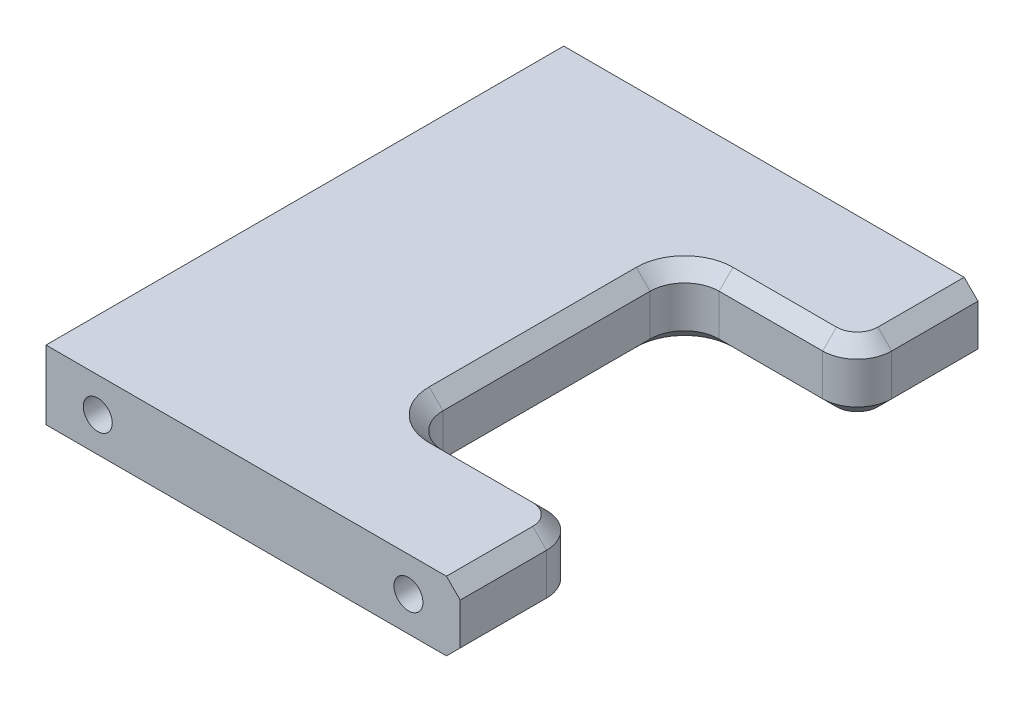
SolidWorks part; units mm, degrees
ref_plane "Front Plane" through (0, 0, 0) normal (0, 0, 1) x (1, 0, 0)
ref_plane "Top Plane" through (0, 0, 0) normal (0, 1, 0) x (1, 0, 0)
ref_plane "Right Plane" through (0, 0, 0) normal (1, 0, 0) x (0, 0, -1)
other "Configuration Table"
sketch "Sketch1" plane through (0, 0, 0) normal (0, 1, 0) x (1, 0, 0)
  line L1 (0, 0) -> (60, 0)
  line L2 (0, 0) -> (0, 75)
  line L3 (0, 75) -> (60, 75)
  line L4 (60, 0) -> (60, 75)
  dimension "D1" = 75
  dimension "D2" = 60
extrude "Boss-Extrude1" add sketch "Sketch1" along normal blind 10
sketch "Sketch5" plane through (0, 0, -75) normal (0, 0, -1) x (-1, 0, 0)
  line L1 (-60, 0) -> (0, 0) construction
  line L2 (-60, 10) -> (-60, 0) construction
  line L3 (0, 10) -> (0, 0) construction
  point P0 (-7.5, 5)
  point P11 (-52.5, 5)
  dimension "D1" = 5
  dimension "D2" = 45
  dimension "D3" = 7.5
  dimension "D4" = 7.5
  dimension "D5" = 5
hole_wizard "M5 Tapped Hole1" positions "Sketch5" profile "Sketch6" tap size "M5" standard "GB"
sketch "Sketch6" plane through (7.5, 5, -75) normal (1, 0, 0) x (0, 1, 0)
  line L0 (0, 0) -> (0, 13.6618)
  line L1 (0, 13.6618) -> (2.1, 12.4)
  line L2 (2.1, 12.4) -> (2.1, 0)
  line L5 (2.1, 0) -> (0, 0)
  line L10 (0, 13.6618) -> (-2.1, 12.4) construction
  line L11 (0, -6.35) -> (0, 107.95) construction
  dimension "螺纹孔钻头直径" = 4.2
  dimension "螺纹孔钻头深度" = 12.4
  dimension "导头角度" = 118
cosmetic thread "Hole thread11" parameters "D1"=10, "D2"=5
cosmetic thread "Hole thread12" parameters "D1"=10, "D2"=5
sketch "Sketch7" plane through (0, 0, 0) normal (0, 0, 1) x (1, 0, 0)
  line L0 (0, 0) -> (60, 0) construction
  line L2 (60, 10) -> (60, 0) construction
  line L3 (0, 10) -> (0, 0) construction
  point P0 (52.5, 5)
  point P1 (7.5, 5)
  dimension "D1" = 5
  dimension "D2" = 45
  dimension "D3" = 7.5
  dimension "D4" = 7.5
hole_wizard "M5 Tapped Hole2" positions "Sketch7" profile "Sketch8" tap size "M5" standard "GB"
sketch "Sketch8" plane through (52.5, 5, 0) normal (1, 0, 0) x (0, -1, 0)
  line L0 (0, 0) -> (0, 13.6618)
  line L1 (0, 13.6618) -> (2.1, 12.4)
  line L2 (2.1, 12.4) -> (2.1, 0)
  line L5 (2.1, 0) -> (0, 0)
  line L10 (0, 13.6618) -> (-2.1, 12.4) construction
  line L11 (0, -6.35) -> (0, 107.95) construction
  dimension "螺纹孔钻头直径" = 4.2
  dimension "螺纹孔钻头深度" = 12.4
  dimension "导头角度" = 118
cosmetic thread "Hole thread5" parameters "D1"=10, "D2"=5
cosmetic thread "Hole thread6" parameters "D1"=10, "D2"=5
sketch "Sketch9" plane through (0, 10, 0) normal (0, 1, 0) x (1, 0, 0)
  line L0 (60, 0) -> (60, 75) construction
  line L1 (35, 57.5) -> (60, 57.5)
  line L2 (35, 57.5) -> (35, 17.5)
  line L3 (35, 17.5) -> (60, 17.5)
  line L4 (60, 57.5) -> (60, 17.5)
  line L6 (0, 37.5) -> (3.1496, 37.5) construction
  line L7 (0, 75) -> (0, 0) construction
  point P13 (35, 37.5)
  dimension "D1" = 25
  dimension "D2" = 40
extrude "Cut-Extrude1" cut sketch "Sketch9" against normal through all
fillet "Fillet1" radius 5 4 edges at (35, 5, -17.5) (35, 5, -57.5) (60, 5, -57.5) (60, 5, -17.5)
chamfer "Chamfer1" distance 2 angle 45 18 edges at (60, 0, -68.75) (60, 0, -6.25) (58.5355, 0, -58.9645) (58.5355, 0, -16.0355) (47.5, 0, -57.5) (47.5, 0, -17.5) (36.4645, 0, -56.0355) (36.4645, 0, -18.9645) (35, 0, -37.5) (60, 10, -68.75) (60, 10, -6.25) (58.5355, 10, -58.9645) (58.5355, 10, -16.0355) (47.5, 10, -57.5) (47.5, 10, -17.5) (36.4645, 10, -56.0355) (36.4645, 10, -18.9645) (35, 10, -37.5)
